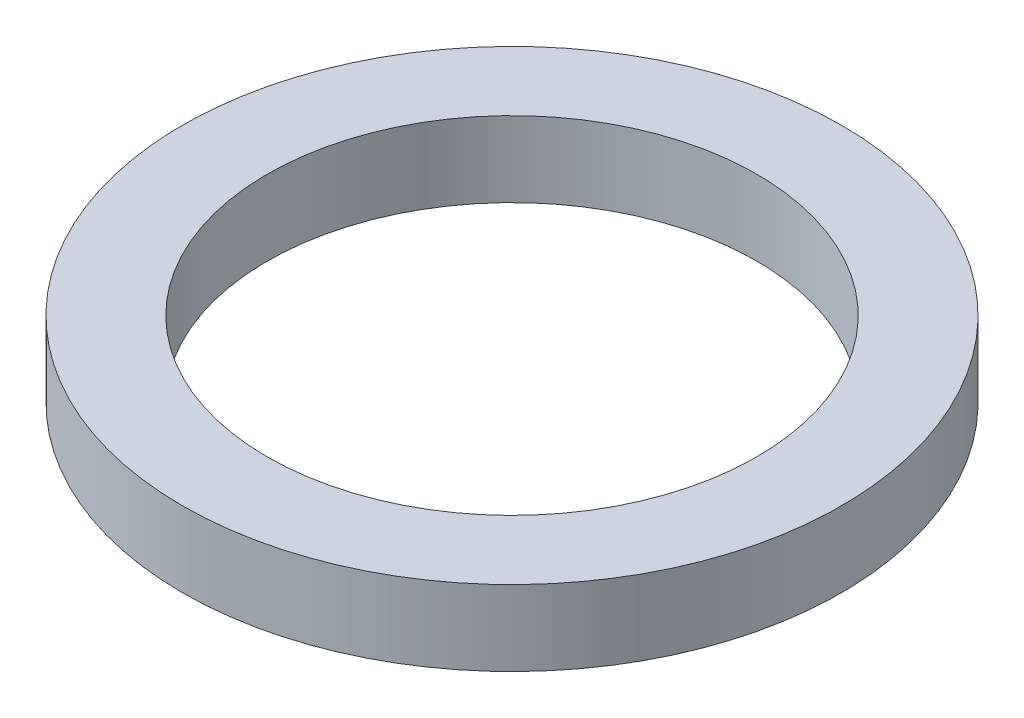
SolidWorks part; units mm, degrees
ref_plane "Front Plane" through (0, 0, 0) normal (0, 0, 1) x (1, 0, 0)
ref_plane "Top Plane" through (0, 0, 0) normal (0, 1, 0) x (1, 0, 0)
ref_plane "Right Plane" through (0, 0, 0) normal (1, 0, 0) x (0, 0, -1)
sketch "Sketch 1" plane through (0, 0, 0) normal (0, 1, 0) x (1, 0, 0)
  circle A0 centre (0, 0) radius 26
  circle A1 centre (0, 0) radius 35
  dimension "D1" = 52
  dimension "D2" = 70
extrude "Boss-Extrude 1" add sketch "Sketch 1" along normal blind 8
